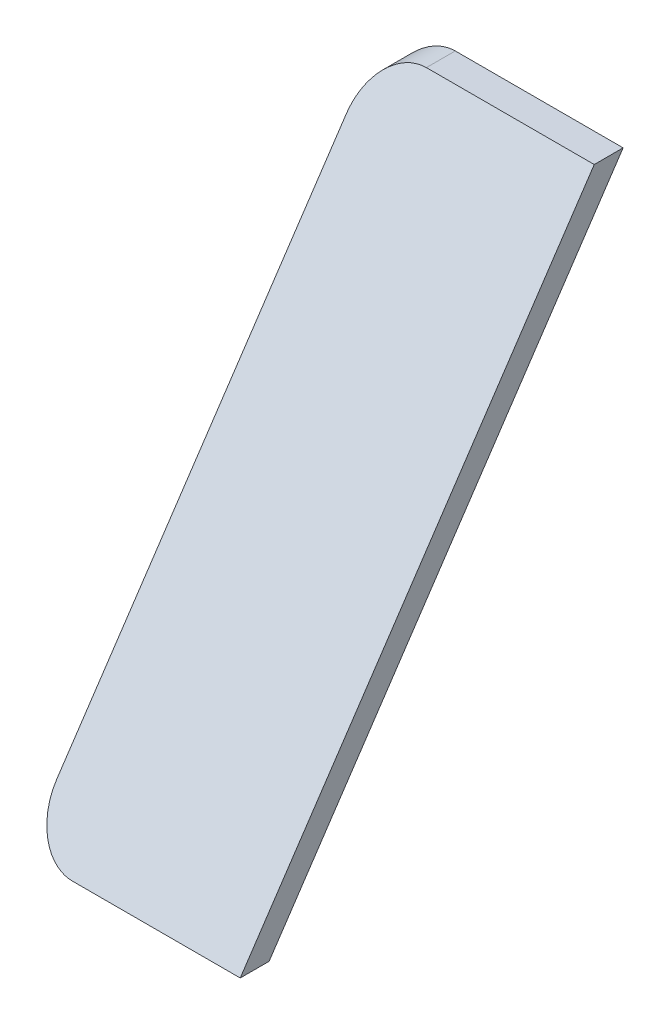
from build123d import *

# Parameters (mm, degrees)
EXTRUDE_2_DEPTH     = 100
SKETCH_3_OUTSIDE_W  = 133.064
SKETCH_3_OUTSIDE_H  = 143.064
CUT_EXTRUDE_5_DEPTH = 100


with BuildPart() as part:
    # 草图1 → 凸台-拉伸2 (new body)
    with BuildSketch(Plane.XY):
        with BuildLine():
            Line((-679.821296296, 67.7), (-679.821296296, -42.3))
            Line((-679.821296296, -42.3), (-714.821296296, -42.3))
            ThreePointArc((-714.821296296, -42.3), (-721.892364108, -39.371067812), (-724.821296296, -32.3))
            Line((-724.821296296, -32.3), (-724.821296296, 57.7))
            ThreePointArc((-724.821296296, 57.7), (-721.892364108, 64.771067812), (-714.821296296, 67.7))
            Line((-714.821296296, 67.7), (-679.821296296, 67.7))
        make_face()
    extrude(amount=EXTRUDE_2_DEPTH)

    # 草图3 outside → 切除-拉伸5 (cut)
    with BuildSketch(Plane(origin=(-679.821296296, 0, 0), x_dir=(0, 0, -1), z_dir=(1, 0, 0))):
        with Locations((-50, 12.7)):
            Rectangle(SKETCH_3_OUTSIDE_W, SKETCH_3_OUTSIDE_H)
        Polygon((-86.021487915, -42.3), (-80, -42.3), (-6.182486595, 67.7), (-12.203974509, 67.7), (-84.151797754, -39.513860124), align=None, mode=Mode.SUBTRACT)
    extrude(amount=-CUT_EXTRUDE_5_DEPTH, mode=Mode.SUBTRACT)


solid = part.part
